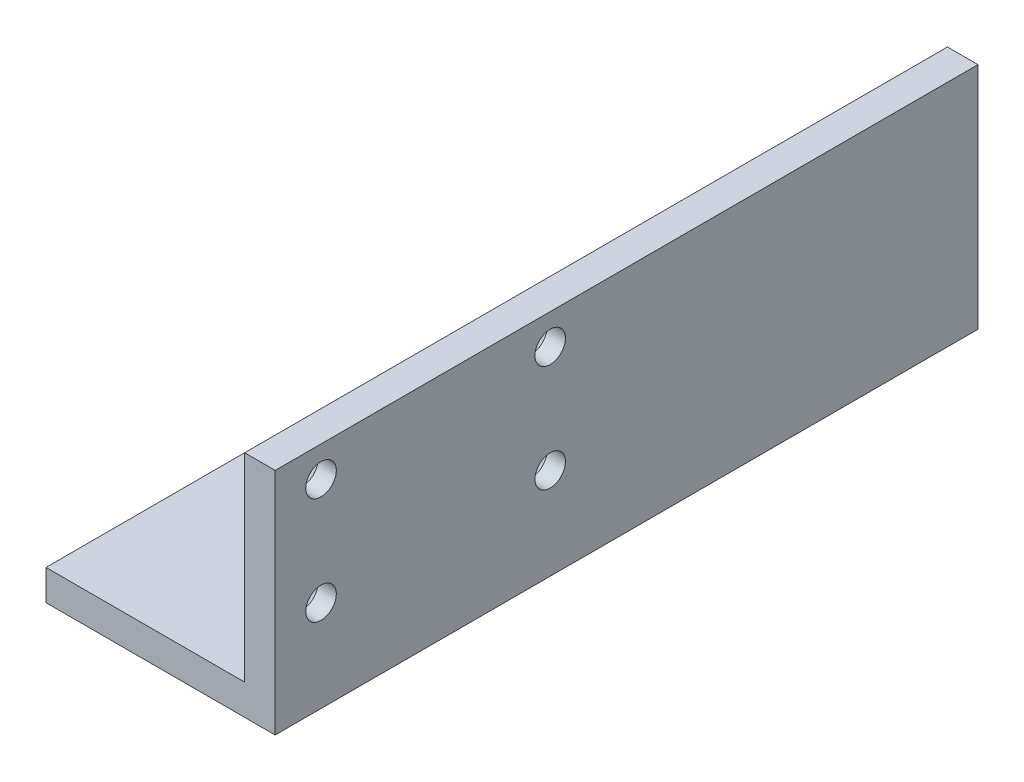
SolidWorks part; units mm, degrees
material "6061Al"
ref_plane "前视基准面" through (0, 0, 0) normal (0, 0, 1) x (1, 0, 0)
ref_plane "上视基准面" through (0, 0, 0) normal (0, 1, 0) x (1, 0, 0)
ref_plane "右视基准面" through (0, 0, 0) normal (1, 0, 0) x (0, 0, -1)
sketch "草图1" plane through (0, 0, 0) normal (0, 0, 1) x (1, 0, 0)
  line L0 (0, 0) -> (75, 0)
  line L1 (75, 0) -> (75, 75)
  line L2 (75, 75) -> (65, 75)
  line L3 (65, 75) -> (65, 10)
  line L4 (65, 10) -> (0, 10)
  line L5 (0, 10) -> (0, 0)
  dimension "D1" = 10
  dimension "D2" = 10
  dimension "D3" = 75
  dimension "D4" = 75
extrude "凸台-拉伸1" add sketch "草图1" along normal mid plane 100
hole_wizard "M8 六角凹锥坑螺钉的锥形沉头孔1" positions "草图2" profile "草图3" countersink size "M8" standard "ISO" end condition through all
sketch "草图2" plane through (65, 0, 0) normal (-1, 0, 0) x (0, 0, 1)
  line L0 (-50, 75) -> (-50, 10) construction
  line L1 (50, 0) -> (-50, 0) construction
  point P0 (-40, 65)
  point P2 (35, 65)
  point P4 (-40, 30)
  point P6 (35, 30)
  dimension "D1" = 75
  dimension "D2" = 10
  dimension "D3" = 35
  dimension "D4" = 30
sketch "草图3" plane through (65, 65, -40) normal (0, 1, 0) x (0, 0, 1)
  line L0 (0, 0) -> (0, 10)
  line L1 (0, 10) -> (5, 10)
  line L2 (5, 10) -> (5, 3.96)
  line L3 (5, 3.96) -> (8.96, 0)
  line L5 (8.96, 0) -> (0, 0)
  line L6 (-5, 3.96) -> (-8.96, 0) construction
  line L11 (0, -6.35) -> (0, 107.95) construction
  dimension "通孔孔直径" = 10
  dimension "通孔孔深度" = 10
  dimension "近端锥形沉头孔直径" = 17.92
  dimension "近端锥形沉头孔角度" = 90
other "移动面1" face at (46.6667, 28.3333, -50) parameters "D1"=130
hole_wizard "M8 间隙孔1" positions "草图4" profile "草图5" hole size "M8" standard "ISO" end condition through all
sketch "草图4" plane through (0, 10, 0) normal (0, 1, 0) x (1, 0, 0)
  line L3 (65, 180) -> (0, 180) construction
  line L4 (65, -50) -> (65, 180) construction
  point P0 (10.5, 165)
  point P2 (10.5, 95)
  point P4 (44.5, 165)
  point P6 (44.5, 95)
  dimension "D1" = 70
  dimension "D2" = 34
  dimension "D3" = 20.5
  dimension "D4" = 15
sketch "草图5" plane through (10.5, 10, -165) normal (1, 0, 0) x (0, 0, 1)
  line L0 (0, 0) -> (0, 10)
  line L1 (0, 10) -> (5, 10)
  line L2 (5, 10) -> (5, 0)
  line L5 (5, 0) -> (0, 0)
  line L11 (0, -6.35) -> (0, 107.95) construction
  dimension "通孔孔直径" = 10
  dimension "通孔孔深度" = 10
